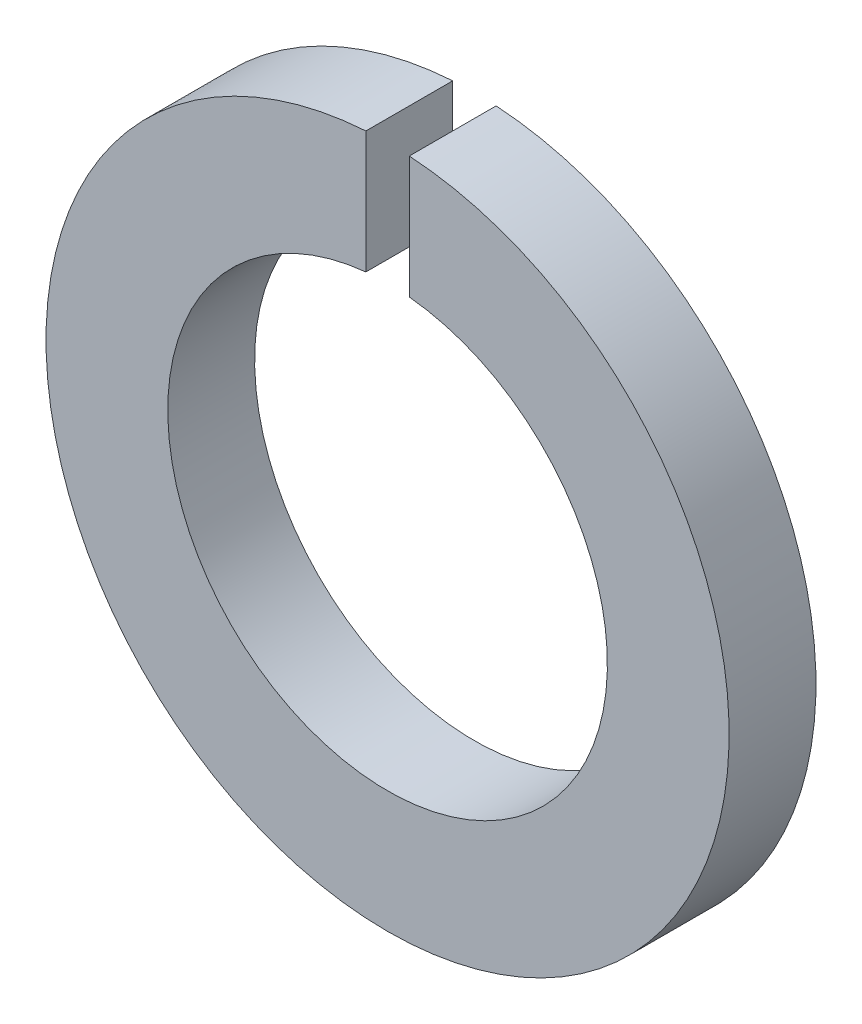
from build123d import *

# Parameters (mm, degrees)
EXTRUDE_1_DEPTH = 3.2


with BuildPart() as part:
    # Sketch 263 → 拉伸1 (new body)
    with BuildSketch(Plane.XY):
        with BuildLine():
            Line((-0.8, 12.560397013), (-0.8, 8.060397013))
            ThreePointArc((-0.8, 8.060397013), (0, -8.1), (0.8, 8.060397013))
            Line((0.8, 8.060397013), (0.8, 12.560397013))
            ThreePointArc((0.8, 12.560397013), (0, -12.585848128), (-0.8, 12.560397013))
        make_face()
    extrude(amount=EXTRUDE_1_DEPTH)


solid = part.part
